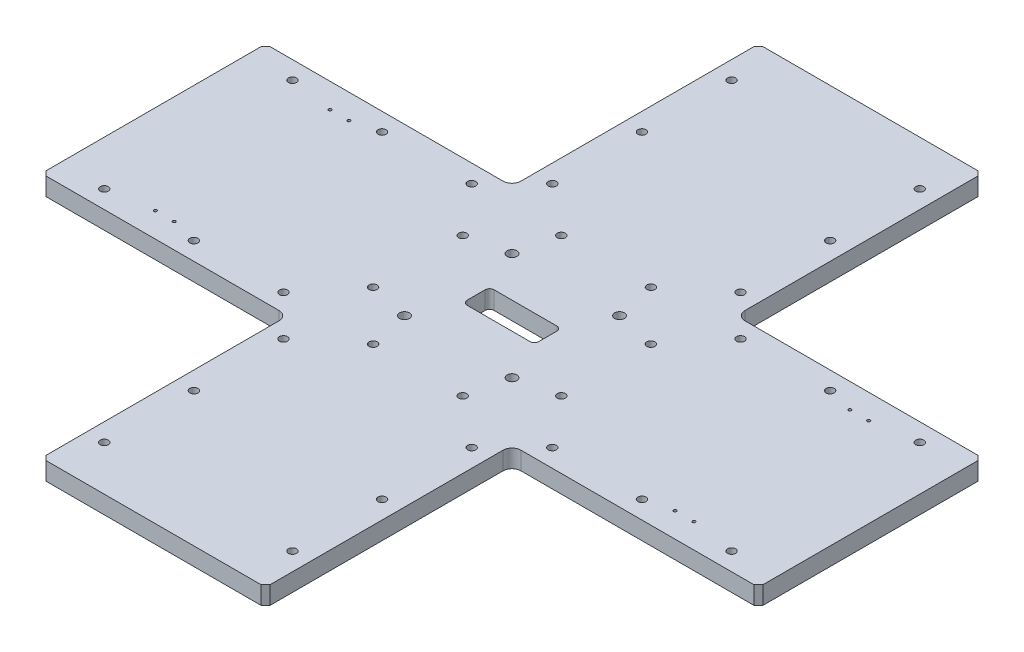
SolidWorks part; units mm, degrees
ref_plane "前视基准面" through (0, 0, 0) normal (0, 0, 1) x (1, 0, 0)
ref_plane "上视基准面" through (0, 0, 0) normal (0, 1, 0) x (1, 0, 0)
ref_plane "右视基准面" through (0, 0, 0) normal (1, 0, 0) x (0, 0, -1)
sketch "草图1" plane through (0, 0, 0) normal (0, 1, 0) x (1, 0, 0)
  line L0 (-125, 125) -> (-125, 400)
  line L1 (-125, -400) -> (125, -400)
  line L2 (-125, -400) -> (-125, -125)
  line L3 (-125, 400) -> (125, 400)
  line L4 (125, -400) -> (125, -125)
  line L5 (-400, 125) -> (-125, 125)
  line L6 (-400, 125) -> (-400, -125)
  line L7 (-400, -125) -> (-125, -125)
  line L8 (400, 125) -> (400, -125)
  line L9 (125, 125) -> (400, 125)
  line L10 (125, 125) -> (125, 400)
  line L11 (125, -125) -> (400, -125)
  line L12 (0, 0) -> (0, 125.7831) construction
  line L13 (0, 0) -> (153.381, 0) construction
  point P8 (0, 400)
  point P12 (-400, 0)
  dimension "D1" = 800
  dimension "D2" = 800
  dimension "D3" = 250
extrude "凸台-拉伸1" add sketch "草图1" along normal blind 20
fillet "圆角1" radius 10 4 edges at (-125, 10, 125) (-125, 10, -125) (125, 10, 125) (125, 10, -125)
chamfer "倒角1" distance 5 angle 45 8 edges at (-125, 10, 400) (125, 10, 400) (400, 10, 125) (400, 10, -125) (125, 10, -400) (-125, 10, -400) (-400, 10, -125) (-400, 10, 125)
sketch "草图2" plane through (0, 0, 0) normal (0, -1, 0) x (1, 0, 0)
  line L1 (-35, 15) -> (35, 15)
  line L2 (-40, 10) -> (-40, -10)
  line L3 (-35, -15) -> (35, -15)
  line L4 (40, 10) -> (40, -10)
  line L5 (-40, 15) -> (40, -15) construction
  line L6 (-40, -15) -> (40, 15) construction
  arc A0 (35, 15) -> (40, 10) centre (35, 10) cw
  arc A1 (-40, -10) -> (-35, -15) centre (-35, -10) ccw
  arc A2 (-35, 15) -> (-40, 10) centre (-35, 10) ccw
  arc A3 (35, -15) -> (40, -10) centre (35, -10) ccw
  point P0 (0, 0)
  dimension "D3" = 5
  dimension "D1" = 30
  dimension "D2" = 80
extrude "切除-拉伸1" cut sketch "草图2" against normal through all
sketch "草图5" plane through (0, 20, 0) normal (0, 1, 0) x (1, 0, 0)
  line L0 (0, 0) -> (0, 86.154) construction
  line L2 (0, 0) -> (72.6237, 0) construction
  point P0 (-60, 60)
  point P12 (60, 60)
  point P14 (60, -60)
  point P15 (-60, -60)
  dimension "D1" = 120
  dimension "D2" = 60
hole_wizard "M10 间隙孔1" positions "草图5" profile "草图4" hole size "M10" standard "GB" end condition through all
sketch "草图4" plane through (-60, 20, -60) normal (1, 0, 0) x (0, 0, 1)
  line L0 (0, 0) -> (0, 20)
  line L1 (0, 20) -> (5.5, 20)
  line L2 (5.5, 20) -> (5.5, 0)
  line L5 (5.5, 0) -> (0, 0)
  line L11 (0, -6.35) -> (0, 107.95) construction
  dimension "通孔孔直径" = 11
  dimension "通孔孔深度" = 20
sketch "草图8" plane through (0, 0, 0) normal (0, -1, 0) x (-1, 0, 0)
  line L1 (256.3287, 0) -> (-256.3287, 0) construction
  line L3 (0, -247.4476) -> (0, 247.4476) construction
  line L5 (-120, 400) -> (120, 400) construction
  line L6 (-125, 135) -> (-125, 395) construction
  line L7 (-400, -120) -> (-400, 120) construction
  line L8 (-395, 125) -> (-135, 125) construction
  point P0 (-105, 350)
  point P2 (-105, 250)
  point P4 (-105, 150)
  point P22 (-105, 50)
  point P33 (-350, 105)
  point P35 (-250, 105)
  point P37 (-150, 105)
  point P39 (-50, 105)
  point P50 (50, 105)
  point P51 (150, 105)
  point P52 (250, 105)
  point P53 (350, 105)
  point P54 (105, 50)
  point P55 (105, 150)
  point P56 (105, 250)
  point P57 (105, 350)
  point P59 (0, 0)
  point P60 (105, -350)
  point P61 (105, -250)
  point P62 (105, -150)
  point P63 (105, -50)
  point P64 (350, -105)
  point P65 (250, -105)
  point P66 (150, -105)
  point P67 (50, -105)
  point P68 (-50, -105)
  point P69 (-150, -105)
  point P70 (-250, -105)
  point P71 (-350, -105)
  point P72 (-105, -50)
  point P73 (-105, -150)
  point P74 (-105, -250)
  point P75 (-105, -350)
  dimension "D1" = 50
  dimension "D2" = 100
  dimension "D3" = 100
  dimension "D4" = 100
  dimension "D5" = 20
  dimension "D6" = 50
  dimension "D7" = 100
  dimension "D8" = 100
  dimension "D9" = 100
  dimension "D10" = 20
hole_wizard "M8 六角圆柱头螺钉的柱形沉头孔1" positions "草图8" profile "草图7" counterbore size "M8" standard "GB" end condition through all
sketch "草图7" plane through (105, 0, -350) normal (1, 0, 0) x (0, 0, -1)
  line L0 (0, 0) -> (0, 20)
  line L1 (0, 20) -> (4.5, 20)
  line L3 (4.5, 20) -> (4.5, 9)
  line L4 (4.5, 9) -> (7.5, 9)
  line L5 (7.5, 9) -> (7.5, 0)
  line L7 (7.5, 0) -> (0, 0)
  line L11 (0, -6.35) -> (0, 107.95) construction
  dimension "通孔孔直径" = 9
  dimension "通孔孔深度" = 20
  dimension "柱形沉头孔直径" = 15
  dimension "柱形沉头孔深度" = 9
sketch "草图11" plane through (0, 0, 0) normal (0, -1, 0) x (-1, 0, 0)
  line L0 (-190.6473, 0) -> (190.6473, 0) construction
  line L2 (0, 0) -> (0, -172.9794) construction
  point P0 (-300.5, 97.5)
  point P3 (-279.5, 97.5)
  point P12 (-279.5, -97.5)
  point P13 (-300.5, -97.5)
  point P19 (300.5, -97.5)
  point P20 (279.5, -97.5)
  point P21 (279.5, 97.5)
  point P22 (300.5, 97.5)
hole_wizard "M4 螺纹孔1" positions "草图11" profile "草图10" tap size "M4" standard "GB" end condition through all
sketch "草图10" plane through (300.5, 0, -97.5) normal (1, 0, 0) x (0, 0, -1)
  line L0 (0, 0) -> (0, 20)
  line L1 (0, 20) -> (1.65, 20)
  line L2 (1.65, 20) -> (1.65, 0)
  line L5 (1.65, 0) -> (0, 0)
  line L11 (0, -6.35) -> (0, 107.95) construction
  dimension "通孔螺纹孔钻头直径" = 3.3
  dimension "通孔螺纹孔钻头深度" = 20
cosmetic thread "孔螺纹线1" parameters "D2"=4
cosmetic thread "孔螺纹线2" parameters "D2"=4
cosmetic thread "孔螺纹线3" parameters "D2"=4
cosmetic thread "孔螺纹线4" parameters "D2"=4
cosmetic thread "孔螺纹线5" parameters "D2"=4
cosmetic thread "孔螺纹线6" parameters "D2"=4
cosmetic thread "孔螺纹线7" parameters "D2"=4
cosmetic thread "孔螺纹线8" parameters "D2"=4
